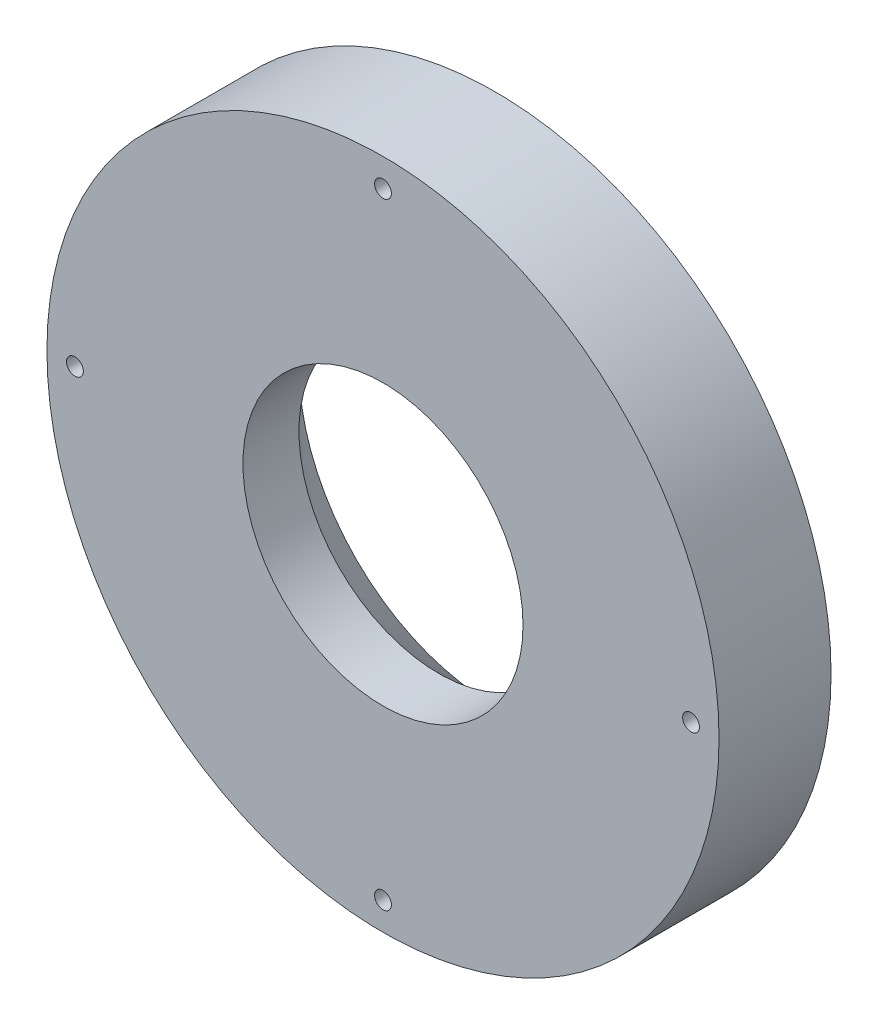
SolidWorks part; units mm, degrees
ref_plane "前视基准面" through (0, 0, 0) normal (0, 0, 1) x (1, 0, 0)
ref_plane "上视基准面" through (0, 0, 0) normal (0, 1, 0) x (1, 0, 0)
ref_plane "右视基准面" through (0, 0, 0) normal (1, 0, 0) x (0, 0, -1)
sketch "草图1" plane through (0, 0, 0) normal (0, 0, 1) x (1, 0, 0)
  circle A0 centre (0, 0) radius 25
  circle A1 centre (0, 0) radius 60
  dimension "D1" = 50
  dimension "D2" = 120
extrude "凸台-拉伸1" add sketch "草图1" along normal blind 20
chamfer "倒角1" distance 10 angle 45 1 edges at (25, 0, 0)
sketch "草图2" plane through (0, 0, 20) normal (0, 0, 1) x (1, 0, 0)
  circle A0 centre (0, 0) radius 55 construction
  circle A1 centre (0, 55) radius 1.5
  circle A2 centre (55, 0) radius 1.5
  circle A3 centre (0, -55) radius 1.5
  circle A4 centre (-55, 0) radius 1.5
  point P14 (0, 0)
  dimension "D1" = 110
  dimension "D2" = 3
  dimension "D3" = 4
extrude "切除-拉伸1" cut sketch "草图2" against normal blind 27
